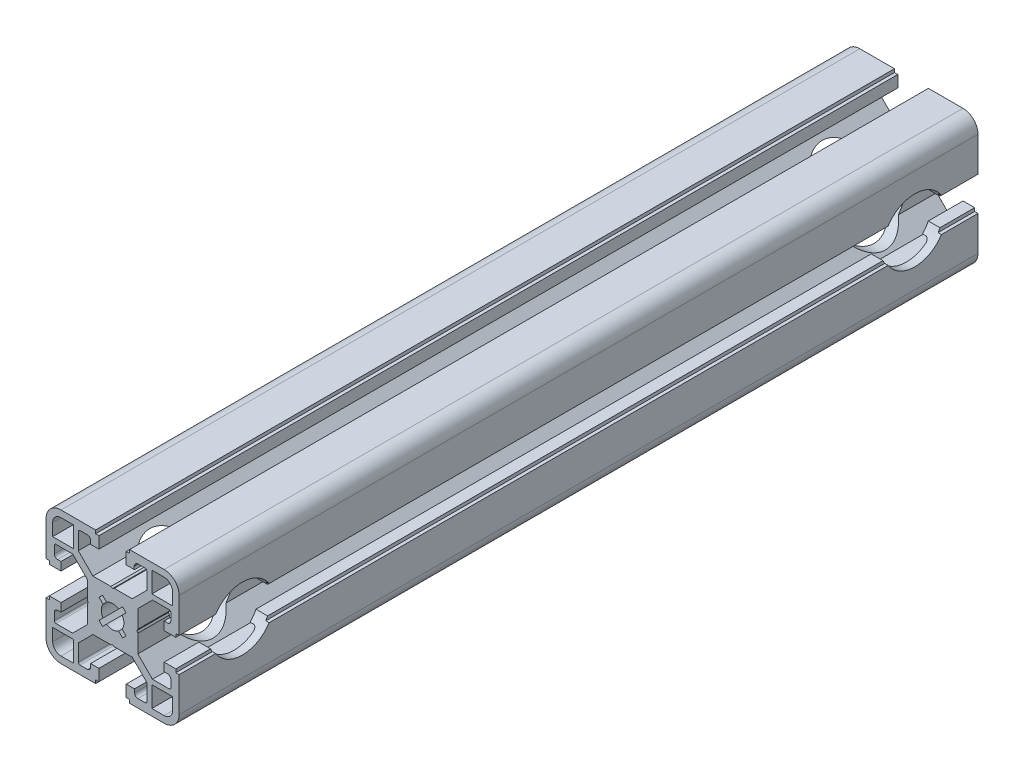
SolidWorks part; units mm, degrees
material "6061 GB/T6892-2006"
ref_plane "前视" through (0, 0, 0) normal (0, 0, 1) x (1, 0, 0)
ref_plane "上视" through (0, 0, 0) normal (0, 1, 0) x (1, 0, 0)
ref_plane "右视" through (0, 0, 0) normal (1, 0, 0) x (0, 0, -1)
sketch "草图1" plane through (0, 0, 0) normal (0, 0, 1) x (1, 0, 0)
  line L0 (-18.9995, -4.1003) -> (-18.9995, -5.1003)
  line L1 (-18.9995, -5.1003) -> (-19.9995, -5.1003)
  line L2 (-19.9995, -5.1003) -> (-19.9995, -15.5003)
  line L3 (-15.4995, -20.0003) -> (-5.0995, -20.0003)
  line L4 (-5.0995, -20.0003) -> (-5.0995, -19.0003)
  line L5 (-5.0995, -19.0003) -> (-4.0995, -19.0003)
  line L6 (-4.0995, -19.0003) -> (-4.0995, -15.5003)
  line L7 (-4.0995, -15.5003) -> (-6.5995, -15.5003)
  line L8 (-6.5995, -15.5003) -> (-6.5995, -16.5003)
  line L9 (-7.5995, -17.5003) -> (-9.7995, -17.5003)
  line L10 (-10.2995, -17.0003) -> (-10.2995, -11.9973)
  line L11 (-10.2995, -11.9973) -> (-5.9025, -7.6003)
  line L12 (-5.9025, -7.6003) -> (-0.5195, -7.6003)
  line L13 (-0.5195, -7.6003) -> (0.0005, -7.3003)
  line L14 (0.0005, -7.3003) -> (0.5195, -7.6003)
  line L15 (0.5195, -7.6003) -> (5.9035, -7.6003)
  line L16 (5.9035, -7.6003) -> (10.3005, -11.9973)
  line L17 (10.3005, -11.9973) -> (10.3005, -17.0003)
  line L18 (9.8005, -17.5003) -> (7.6005, -17.5003)
  line L19 (6.6005, -16.5003) -> (6.6005, -15.5003)
  line L20 (6.6005, -15.5003) -> (4.1005, -15.5003)
  line L21 (4.1005, -15.5003) -> (4.1005, -19.0003)
  line L22 (4.1005, -19.0003) -> (5.1005, -19.0003)
  line L23 (5.1005, -19.0003) -> (5.1005, -20.0003)
  line L24 (5.1005, -20.0003) -> (15.5005, -20.0003)
  line L25 (20.0005, -15.5003) -> (20.0005, -5.1003)
  line L26 (20.0005, -5.1003) -> (19.0005, -5.1003)
  line L27 (19.0005, -5.1003) -> (19.0005, -4.1003)
  line L28 (19.0005, -4.1003) -> (15.5005, -4.1003)
  line L29 (15.5005, -4.1003) -> (15.5005, -6.6003)
  line L30 (15.5005, -6.6003) -> (16.5005, -6.6003)
  line L31 (17.5005, -7.6003) -> (17.5005, -9.8003)
  line L32 (17.0005, -10.3003) -> (11.9975, -10.3003)
  line L33 (11.9975, -10.3003) -> (7.6005, -5.9033)
  line L34 (7.6005, -5.9033) -> (7.6005, -0.5203)
  line L35 (7.6005, -0.5203) -> (7.3005, -0.0003)
  line L36 (7.3005, -0.0003) -> (7.6005, 0.5197)
  line L37 (7.6005, 0.5197) -> (7.6005, 5.9027)
  line L38 (7.6005, 5.9027) -> (11.9975, 10.2997)
  line L39 (11.9975, 10.2997) -> (17.0005, 10.2997)
  line L40 (17.5005, 9.7997) -> (17.5005, 7.5997)
  line L41 (16.5005, 6.5997) -> (15.5005, 6.5997)
  line L42 (15.5005, 6.5997) -> (15.5005, 4.0997)
  line L43 (15.5005, 4.0997) -> (19.0005, 4.0997)
  line L44 (19.0005, 4.0997) -> (19.0005, 5.0997)
  line L45 (19.0005, 5.0997) -> (20.0005, 5.0997)
  line L46 (20.0005, 5.0997) -> (20.0005, 15.4997)
  line L47 (15.5005, 19.9997) -> (5.1005, 19.9997)
  line L48 (5.1005, 19.9997) -> (5.1005, 18.9997)
  line L49 (5.1005, 18.9997) -> (4.1005, 18.9997)
  line L50 (4.1005, 18.9997) -> (4.1005, 15.4997)
  line L51 (4.1005, 15.4997) -> (6.6005, 15.4997)
  line L52 (7.6005, 17.4997) -> (9.8005, 17.4997)
  line L53 (10.3005, 16.9997) -> (10.3005, 11.9967)
  line L54 (10.3005, 11.9967) -> (5.9035, 7.5997)
  line L55 (5.9035, 7.5997) -> (0.5195, 7.5997)
  line L56 (0.5195, 7.5997) -> (0.0005, 7.2997)
  line L57 (0.0005, 7.2997) -> (-0.5195, 7.5997)
  line L58 (-0.5195, 7.5997) -> (-5.9025, 7.5997)
  line L59 (-5.9025, 7.5997) -> (-10.2995, 11.9967)
  line L60 (-10.2995, 11.9967) -> (-10.2995, 16.9997)
  line L61 (-9.7995, 17.4997) -> (-7.5995, 17.4997)
  line L62 (-6.5995, 16.4997) -> (-6.5995, 15.4997)
  line L63 (-6.5995, 15.4997) -> (-4.0995, 15.4997)
  line L64 (-4.0995, 15.4997) -> (-4.0995, 18.9997)
  line L65 (-4.0995, 18.9997) -> (-5.0995, 18.9997)
  line L66 (-5.0995, 18.9997) -> (-5.0995, 19.9997)
  line L67 (-5.0995, 19.9997) -> (-15.4995, 19.9997)
  line L68 (-19.9995, 15.4997) -> (-19.9995, 5.0997)
  line L69 (-19.9995, 5.0997) -> (-18.9995, 5.0997)
  line L70 (-18.9995, 5.0997) -> (-18.9995, 4.0997)
  line L71 (-18.9995, 4.0997) -> (-15.4995, 4.0997)
  line L72 (-15.4995, 4.0997) -> (-15.4995, 6.5997)
  line L73 (-15.4995, 6.5997) -> (-16.4995, 6.5997)
  line L74 (-17.4995, 7.5997) -> (-17.4995, 9.7997)
  line L75 (-16.9995, 10.2997) -> (-11.9965, 10.2997)
  line L76 (-11.9965, 10.2997) -> (-7.5995, 5.9027)
  line L77 (-7.5995, 5.9027) -> (-7.5995, 0.5197)
  line L78 (-7.5995, 0.5197) -> (-7.2995, -0.0003)
  line L79 (-7.2995, -0.0003) -> (-7.5995, -0.5203)
  line L80 (-7.5995, -0.5203) -> (-7.5995, -5.9033)
  line L81 (-7.5995, -5.9033) -> (-11.9965, -10.3003)
  line L82 (-11.9965, -10.3003) -> (-16.9995, -10.3003)
  line L83 (-17.4995, -9.8003) -> (-17.4995, -7.6003)
  line L84 (-16.4995, -6.6003) -> (-15.4995, -6.6003)
  line L85 (-15.4995, -6.6003) -> (-15.4995, -4.1003)
  line L86 (-15.4995, -4.1003) -> (-18.9995, -4.1003)
  line L87 (15.5005, -18.0003) -> (11.8005, -18.0003)
  line L88 (11.8005, -18.0003) -> (11.8005, -11.8003)
  line L89 (11.8005, -11.8003) -> (18.0005, -11.8003)
  line L90 (18.0005, -11.8003) -> (18.0005, -15.5003)
  line L91 (18.0005, 11.7997) -> (11.8005, 11.7997)
  line L92 (11.8005, 11.7997) -> (11.8005, 17.9997)
  line L93 (11.8005, 17.9997) -> (15.5005, 17.9997)
  line L94 (18.0005, 15.4997) -> (18.0005, 11.7997)
  line L95 (-1.8145, -2.8753) -> (-3.0044, -4.0665)
  line L96 (-3.0044, -4.0665) -> (-4.0656, -3.0052)
  line L97 (-4.0656, -3.0052) -> (-2.8745, -1.8153)
  line L98 (-2.8745, 1.8147) -> (-4.0644, 3.0058)
  line L99 (-4.0644, 3.0058) -> (-3.0044, 4.0658)
  line L100 (-3.0044, 4.0658) -> (-1.8145, 2.8747)
  line L101 (1.8145, 2.8747) -> (3.0055, 4.0657)
  line L102 (3.0055, 4.0657) -> (4.0666, 3.0045)
  line L103 (4.0666, 3.0045) -> (2.8755, 1.8147)
  line L104 (2.8755, -1.8153) -> (4.0666, -3.0052)
  line L105 (4.0666, -3.0052) -> (3.0055, -4.0663)
  line L106 (3.0055, -4.0663) -> (1.8145, -2.8753)
  line L107 (-17.9995, -15.5003) -> (-17.9995, -11.8003)
  line L108 (-17.9995, -11.8003) -> (-11.7995, -11.8003)
  line L109 (-11.7995, -11.8003) -> (-11.7995, -18.0003)
  line L110 (-11.7995, -18.0003) -> (-15.4995, -18.0003)
  line L111 (-11.7995, 17.9997) -> (-11.7995, 11.7997)
  line L112 (-11.7995, 11.7997) -> (-17.9995, 11.7997)
  line L113 (-17.9995, 11.7997) -> (-17.9995, 15.4997)
  line L114 (-15.4995, 17.9997) -> (-11.7995, 17.9997)
  arc A0 (-19.9995, -15.5003) -> (-15.4995, -20.0003) centre (-15.4995, -15.5003) ccw
  arc A1 (-6.5995, -16.5003) -> (-7.5995, -17.5003) centre (-7.5995, -16.5003) cw
  arc A2 (-9.7995, -17.5003) -> (-10.2995, -17.0003) centre (-9.7995, -17.0003) cw
  arc A3 (10.3005, -17.0003) -> (9.8005, -17.5003) centre (9.8005, -17.0003) cw
  arc A4 (7.6005, -17.5003) -> (6.6005, -16.5003) centre (7.6005, -16.5003) cw
  arc A5 (15.5005, -20.0003) -> (20.0005, -15.5003) centre (15.5005, -15.5003) ccw
  arc A6 (16.5005, -6.6003) -> (17.5005, -7.6003) centre (16.5005, -7.6003) cw
  arc A7 (17.5005, -9.8003) -> (17.0005, -10.3003) centre (17.0005, -9.8003) cw
  arc A8 (17.0005, 10.2997) -> (17.5005, 9.7997) centre (17.0005, 9.7997) cw
  arc A9 (17.5005, 7.5997) -> (16.5005, 6.5997) centre (16.5005, 7.5997) cw
  arc A10 (20.0005, 15.4997) -> (15.5005, 19.9997) centre (15.5005, 15.4997) ccw
  arc A11 (6.6005, 15.4997) -> (6.6005, 16.4997) centre (7.1003, 15.9997) cw
  arc A12 (6.6005, 16.4997) -> (7.6005, 17.4997) centre (7.6005, 16.4997) cw
  arc A13 (9.8005, 17.4997) -> (10.3005, 16.9997) centre (9.8005, 16.9997) cw
  arc A14 (-10.2995, 16.9997) -> (-9.7995, 17.4997) centre (-9.7995, 16.9997) cw
  arc A15 (-7.5995, 17.4997) -> (-6.5995, 16.4997) centre (-7.5995, 16.4997) cw
  arc A16 (-15.4995, 19.9997) -> (-19.9995, 15.4997) centre (-15.4995, 15.4997) ccw
  arc A17 (-16.4995, 6.5997) -> (-17.4995, 7.5997) centre (-16.4995, 7.5997) cw
  arc A18 (-17.4995, 9.7997) -> (-16.9995, 10.2997) centre (-16.9995, 9.7997) cw
  arc A19 (-16.9995, -10.3003) -> (-17.4995, -9.8003) centre (-16.9995, -9.8003) cw
  arc A20 (-17.4995, -7.6003) -> (-16.4995, -6.6003) centre (-16.4995, -7.6003) cw
  arc A21 (18.0005, -15.5003) -> (15.5005, -18.0003) centre (15.5005, -15.5003) cw
  arc A22 (15.5005, 17.9997) -> (18.0005, 15.4997) centre (15.5005, 15.4997) cw
  arc A23 (-2.8745, -1.8153) -> (-2.8745, 1.8147) centre (0.0005, -0.0003) cw
  arc A24 (-1.8145, 2.8747) -> (1.8145, 2.8747) centre (0, -0.0007) cw
  arc A25 (2.8755, 1.8147) -> (2.8755, -1.8153) centre (0.0005, -0.0003) cw
  arc A26 (1.8145, -2.8753) -> (-1.8145, -2.8753) centre (0, 0) cw
  arc A27 (-15.4995, -18.0003) -> (-17.9995, -15.5003) centre (-15.4995, -15.5003) cw
  arc A28 (-17.9995, 15.4997) -> (-15.4995, 17.9997) centre (-15.4995, 15.4997) cw
extrude "凸台-拉伸1" add sketch "草图1" against normal blind 240
hole_wizard "Ø19.0 (19) 直径孔1" positions "草图2" profile "草图3" hole size "Ø19.0" standard "GB" end condition through all
sketch "草图2" plane through (20.0005, 0, 0) normal (1, 0, 0) x (0, 0, -1)
  line L0 (240, -0.0003) -> (0, -0.0003) construction
  point P0 (19, -0.0003)
  point P4 (221, -0.0003)
  dimension "D1" = 19
  dimension "D2" = 19
sketch "草图3" plane through (20.0005, -0.0003, -19) normal (0, 1, 0) x (0, 0, -1)
  line L0 (0, 0) -> (0, 40)
  line L1 (0, 40) -> (9.5, 40)
  line L2 (9.5, 40) -> (9.5, 0)
  line L5 (9.5, 0) -> (0, 0)
  line L11 (0, -6.35) -> (0, 107.95) construction
  dimension "通孔孔直径" = 19
  dimension "通孔孔深度" = 40
